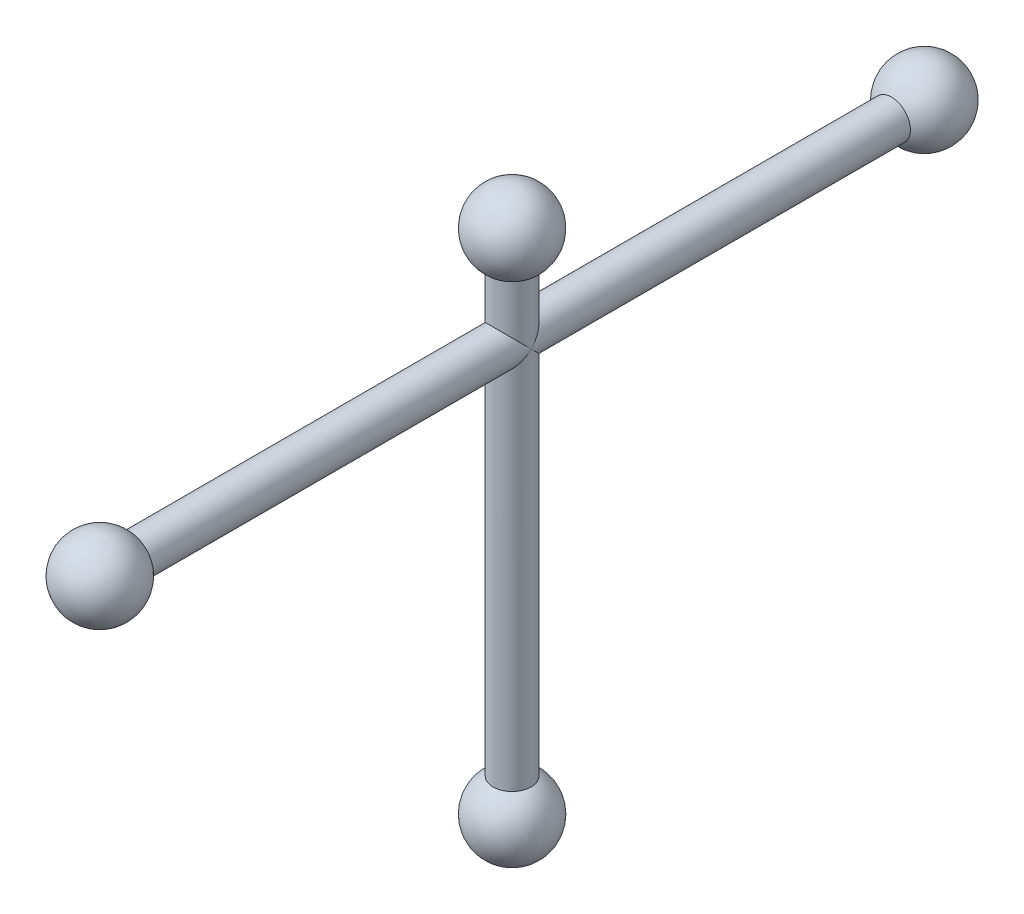
SolidWorks part; units mm, degrees
ref_plane "Front Plane" through (0, 0, 0) normal (0, 0, 1) x (1, 0, 0)
ref_plane "Top Plane" through (0, 0, 0) normal (0, 1, 0) x (1, 0, 0)
ref_plane "Right Plane" through (0, 0, 0) normal (1, 0, 0) x (0, 0, -1)
sketch "Sketch1" plane through (0, 0, 0) normal (0, 0, 1) x (1, 0, 0)
  circle A0 centre (0, 0) radius 15
  dimension "D1" = 30
extrude "Boss-Extrude1" add sketch "Sketch1" along normal mid plane 600
sketch "Sketch2" plane through (0, 0, 0) normal (0, 1, 0) x (1, 0, 0)
  line L0 (0, 355) -> (0, 295)
  line L1 (0, 0) -> (0, 325) construction
  line L2 (15, 300) -> (-15, 300) construction
  arc A0 (0, 295) -> (0, 355) centre (0, 325) ccw
  dimension "D1" = 60
  dimension "D2" = 25
revolve "Revolve1" add sketch "Sketch2" angle 360 about L0
mirror "Mirror1" about plane through (0, 0, 0) normal (0, 0, 1) of "Revolve1"
sketch "Sketch3" plane through (0, 0, 0) normal (0, 1, 0) x (1, 0, 0)
  circle A0 centre (0, 0) radius 15
extrude "Boss-Extrude2" add sketch "Sketch3" along normal blind 50
sketch "Sketch4" plane through (0, 0, 0) normal (0, 0, 1) x (1, 0, 0)
  line L0 (15, 50) -> (-15, 50) construction
  line L1 (0, 105) -> (0, 45)
  arc A0 (0, 45) -> (0, 105) centre (0, 75) ccw
  dimension "D1" = 60
  dimension "D2" = 25
revolve "Revolve2" add sketch "Sketch4" angle 360 about L1
sketch "Sketch5" plane through (0, 0, 0) normal (0, 1, 0) x (1, 0, 0)
  circle A0 centre (0, 0) radius 15
  dimension "D1" = 30
extrude "Boss-Extrude3" add sketch "Sketch5" against normal blind 300
sketch "Sketch6" plane through (0, 0, 0) normal (1, 0, 0) x (0, 0, -1)
  line L0 (0, -295) -> (0, -355)
  line L1 (-15, -300) -> (15, -300) construction
  arc A0 (0, -295) -> (0, -355) centre (0, -325) ccw
  dimension "D2" = 60
  dimension "D1" = 25
sketch "Sketch7" plane through (0, 0, 0) normal (0, 0, 1) x (1, 0, 0)
  circle A0 centre (0, -425) radius 15
  dimension "D1" = 30
revolve "Revolve3" add sketch "Sketch6" angle 360 about L0
